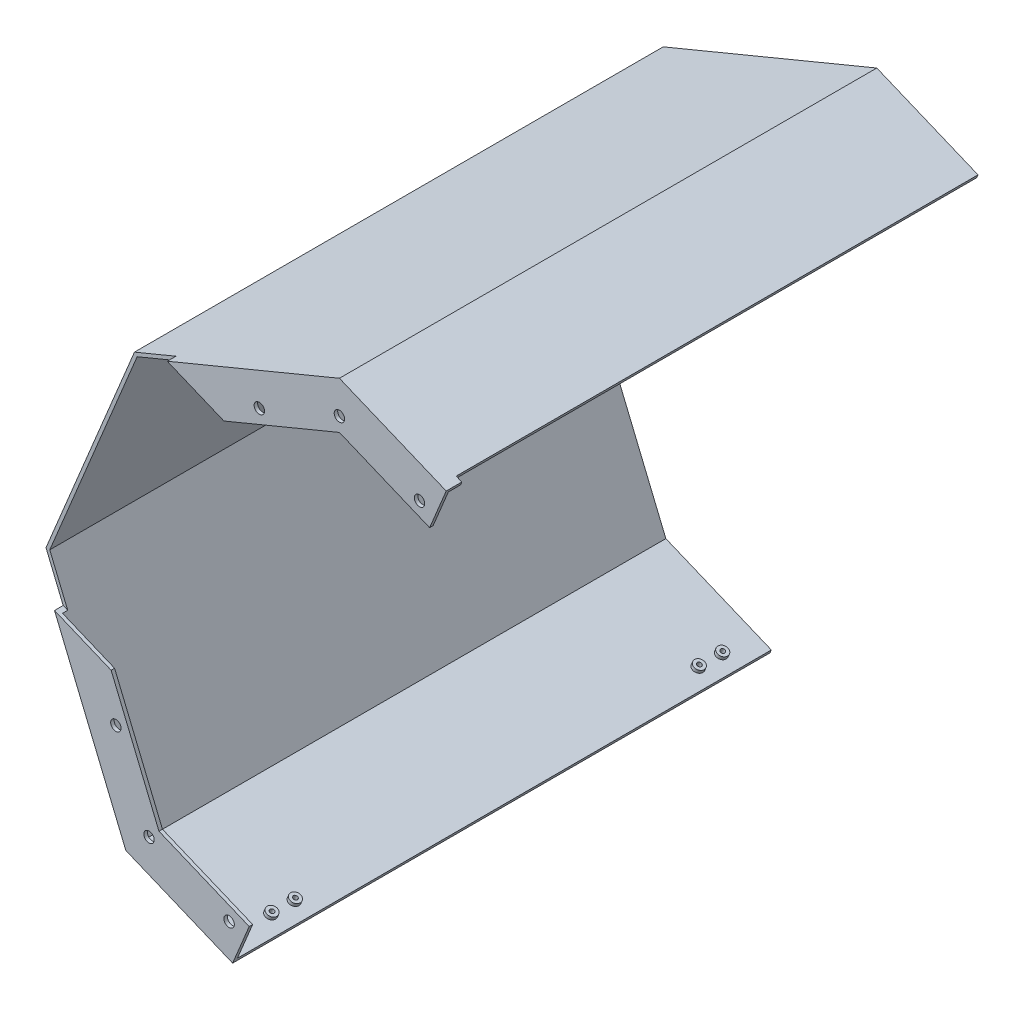
from build123d import *

# Parameters (mm, degrees)
BOSS_EXTRUDE1_DEPTH   = 310
SHELL1_T              = -2
CUT_EXTRUDE1_DEPTH    = 10
CUT_EXTRUDE2_DEPTH    = 397.026111511
CUT_EXTRUDE3_DEPTH    = 5
SKETCH5_R             = 3
CUT_EXTRUDE4_DEPTH    = 10
SKETCH10_R            = 3
BOSS_EXTRUDE3_DEPTH   = 2
M3_TAPPED_HOLE1_D     = 2.5
M3_TAPPED_HOLE1_DEPTH = 4
CUT_EXTRUDE5_REACH    = 492.141
SKETCH17_W            = 3.5
SKETCH17_H            = 301


with BuildPart() as part:
    # Sketch1 → Boss-Extrude1 (new body)
    with BuildSketch(Plane.XY):
        Polygon((-174.265144247, 0), (-123.224065222, -123.224065222), (0, -174.265144247), (123.224065222, -123.224065222), (174.265144247, 0), (123.224065222, 123.224065222), (0, 174.265144247), (-123.224065222, 123.224065222), align=None)
    extrude(amount=BOSS_EXTRUDE1_DEPTH)

    # Shell1
    shell1_openings = [part.faces().sort_by_distance(p)[0] for p in [
        (0, 0, 0),
    ]]
    offset(amount=SHELL1_T, openings=shell1_openings, kind=Kind.INTERSECTION)

    # Sketch2 → Cut-Extrude1 (cut)
    with BuildSketch(Plane.XY.offset(310)):
        Polygon((104.089893603, 104.089893603), (0, 147.20533924), (-104.089893603, 104.089893603), (-147.20533924, 0), (-104.089893603, -104.089893603), (0, -147.20533924), (104.089893603, -104.089893603), (147.20533924, 0), align=None)
    extrude(amount=-CUT_EXTRUDE1_DEPTH, mode=Mode.SUBTRACT)

    # Sketch3 → Cut-Extrude2 (cut, through all)
    with BuildSketch(Plane.XY.offset(310)):
        Polygon((70.138181093, 169.328548035), (-63.801020235, -154.029288344), (130.028007017, -234.315900213), (263.967208344, 89.041936166), align=None)
    extrude(amount=-CUT_EXTRUDE2_DEPTH, mode=Mode.SUBTRACT)

    # Sketch4 → Cut-Extrude3 (cut)
    with BuildSketch(Plane.XY.offset(310)):
        Polygon((-143.932898959, 151.622295845), (-51.544945707, 113.353952609), (-116.60112921, -43.705567918), (-208.989082461, -5.437224682), align=None)
    extrude(amount=-CUT_EXTRUDE3_DEPTH, mode=Mode.SUBTRACT)

    # Sketch5 → Cut-Extrude4 (cut)
    with BuildSketch(Plane.XY.offset(310)):
        with Locations((0, 155.323280742)):
            Circle(SKETCH5_R)
        with Locations((-46.193976626, 136.189109124)):
            Circle(SKETCH5_R)
        with Locations((46.193976626, 136.189109124)):
            Circle(SKETCH5_R)
        with Locations((-128.964316707, -63.636168463)):
            Circle(SKETCH5_R)
        with Locations((-109.830145089, -109.830145089)):
            Circle(SKETCH5_R)
        with Locations((-63.636168463, -128.964316707)):
            Circle(SKETCH5_R)
    extrude(amount=-CUT_EXTRUDE4_DEPTH, mode=Mode.SUBTRACT)

    # Sketch10 → Boss-Extrude3 (add)
    with BuildSketch(Plane(origin=(-60.846665746, -146.896845669, 0), x_dir=(0.9238795325112958, -0.3826834323650679, 0), z_dir=(0.3826834323650679, 0.9238795325112958, 0))):
        with Locations(Location((-9.5, -280, 0), (0, 0, 180))):
            Circle(SKETCH10_R)
        with Locations(Location((-9.5, -266.5, 0), (0, 0, 180))):
            Circle(SKETCH10_R)
        with Locations(Location((-9.5, -33.5, 0), (0, 0, 180))):
            Circle(SKETCH10_R)
        with Locations(Location((-9.5, -20, 0), (0, 0, 180))):
            Circle(SKETCH10_R)
    extrude(amount=BOSS_EXTRUDE3_DEPTH)

    # M3 Tapped Hole1
    with Locations(Plane(origin=(-61.612032611, -148.744604734, 0), x_dir=(-0.9238795325112958, 0.3826834323650679, 0), z_dir=(-0.3826834323650679, -0.9238795325112958, 0))):
        with Locations((9.5, -280), (9.5, -266.5), (9.5, -33.5), (9.5, -20)):
            Hole(M3_TAPPED_HOLE1_D / 2, depth=M3_TAPPED_HOLE1_DEPTH)

    # Sketch17 → Cut-Extrude5 (cut, up to next)
    with BuildSketch(Plane(origin=(61.612032611, 148.744604734, 0), x_dir=(0.923879532511296, -0.38268343236506785, 0), z_dir=(0.38268343236506785, 0.923879532511296, 0)), mode=Mode.PRIVATE) as cut_extrude5_sk1:
        with Locations((-1.75, -150.5)):
            Rectangle(SKETCH17_W, SKETCH17_H)
    cut_extrude5_tool1 = extrude(cut_extrude5_sk1.sketch, amount=-CUT_EXTRUDE5_REACH, mode=Mode.PRIVATE) & part.part
    add(cut_extrude5_tool1.solids().sort_by_distance((59.995243, 149.414301, 150.5))[0], mode=Mode.SUBTRACT)


solid = part.part
